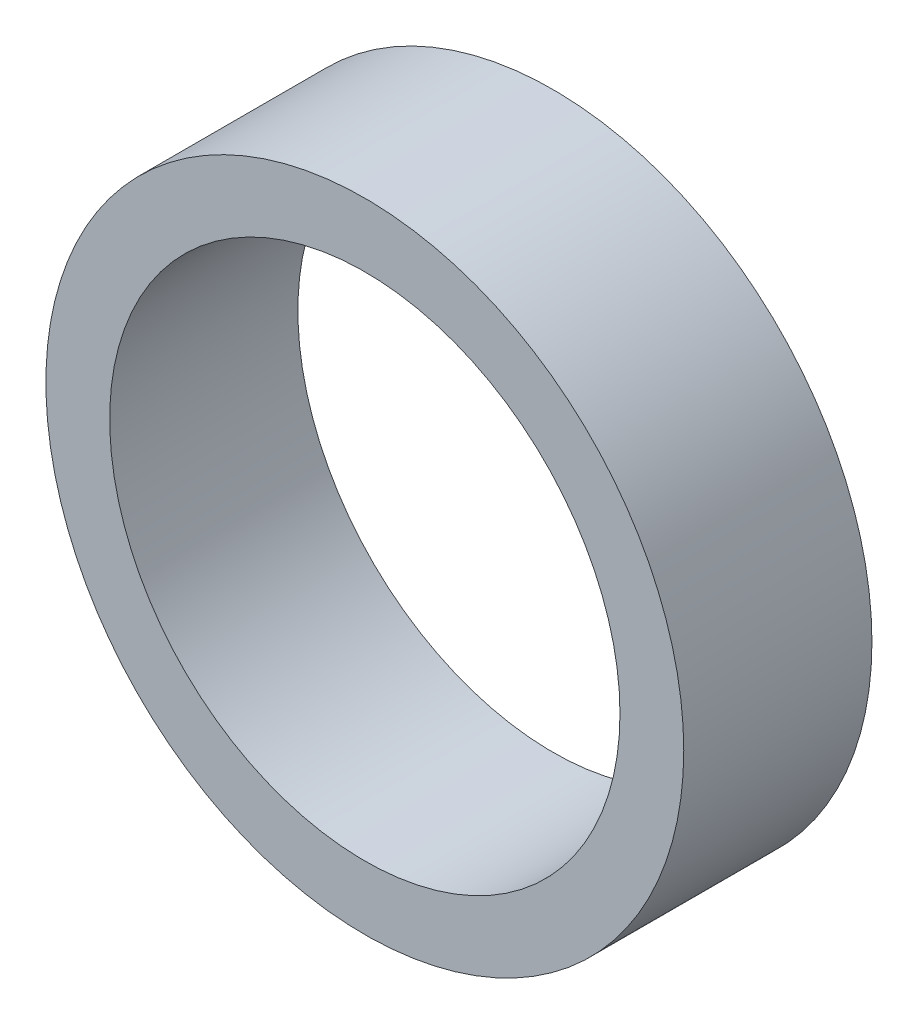
from build123d import *

# Parameters (mm, degrees)
SKETCH1_R           = 50
SKETCH1_R_2         = 40
BOSS_EXTRUDE1_DEPTH = 29.5


with BuildPart() as part:
    # Sketch1 → Boss-Extrude1 (new body)
    with BuildSketch(Plane.XY):
        Circle(SKETCH1_R)
        Circle(SKETCH1_R_2, mode=Mode.SUBTRACT)
    extrude(amount=BOSS_EXTRUDE1_DEPTH)


solid = part.part
